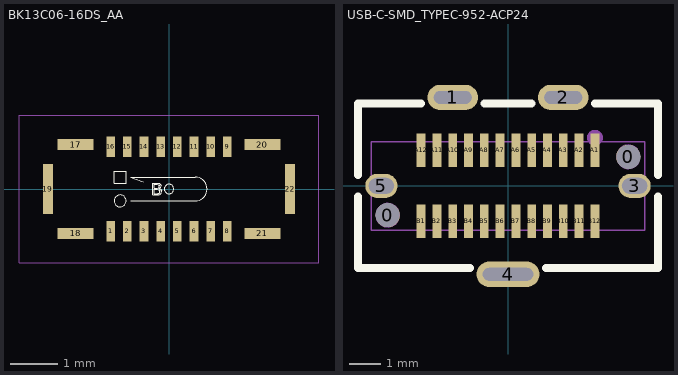
[diagram p0: the footprints below, top view; thin cyan lines are the x and y axes]
# Altium footprint library MISC89352.PcbLib: 2 footprints
Each footprint in its own frame and in the unit in brackets; x right, y up, seen from the top. Pads: shape width x height; smd on the part's side, far side on the other; paste and mask are expansions set on the pad; w line width, h text height; cw(c..) or ccw(c..) is an arc to the next point about the centre after c.

## BK13C06-16DS_AA [mm]
pads (22):
  rect 0.18x0.425 smd paste+0.102 mask+0.072: 1(-1.225,-0.887) 2(-0.875,-0.887) 3(-0.525,-0.887) 4(-0.175,-0.887) 5(0.175,-0.887) 6(0.525,-0.887) 7(0.875,-0.887) 8(1.225,-0.887) 9(1.225,0.887) 10(0.875,0.887) 11(0.525,0.887) 12(0.175,0.887) 13(-0.175,0.887) 14(-0.525,0.887) 15(-0.875,0.887) 16(-1.225,0.887)
  rect 0.75x0.235 smd paste+0.102 mask+0.05: 17(-1.96,0.932) 18(-1.96,-0.932) 20(1.96,0.932) 21(1.96,-0.932)
  rect 0.215x1.04 smd paste+0.102 mask+0.05: 19(-2.54,0) 22(2.54,0)
Top Overlay:
  circle w0.013: c-1.025,-0.25 r0.125
  circle w0.013: c0,0 r0.1
  lines w0.013: -0.8,-0.25 0.55,-0.25 ccw(c0.55,0) 0.55,0.25 -0.8,0.25 -0.537,0.155 ; -1.15,0.125 -0.9,0.125 -0.9,0.375 -1.15,0.375 -1.15,0.125 ; -0.344,-0.125 -0.237,-0.125 -0.217,-0.123 -0.209,-0.121 -0.201,-0.119 -0.187,-0.113 -0.181,-0.108 -0.176,-0.104 -0.167,-0.093 -0.159,-0.078 -0.156,-0.061 -0.156,-0.042 -0.162,-0.023 -0.168,-0.015 -0.174,-0.007 -0.191,0.005 -0.203,0.008 -0.194,0.012 -0.181,0.024 -0.176,0.031 -0.172,0.038 -0.168,0.053 -0.168,0.07 -0.173,0.086 -0.178,0.094 -0.182,0.102 -0.196,0.114 -0.205,0.117 -0.213,0.121 -0.236,0.125 -0.344,0.125 -0.344,-0.125 ; -0.311,-0.095 -0.311,-0.01 -0.242,-0.01 -0.223,-0.012 -0.217,-0.014 -0.211,-0.016 -0.201,-0.023 -0.197,-0.028 -0.193,-0.033 -0.19,-0.046 -0.19,-0.058 -0.192,-0.069 -0.195,-0.074 -0.197,-0.078 -0.204,-0.085 -0.207,-0.087 -0.211,-0.09 -0.221,-0.093 -0.227,-0.094 -0.23,-0.095 -0.241,-0.095 -0.311,-0.095 ; -0.311,0.02 -0.311,0.095 -0.248,0.095 -0.229,0.094 -0.223,0.092 -0.218,0.09 -0.209,0.084 -0.206,0.079 -0.203,0.074 -0.2,0.063 -0.2,0.051 -0.203,0.04 -0.21,0.031 -0.219,0.025 -0.226,0.023 -0.23,0.021 -0.246,0.02 -0.311,0.02
Mechanical 1:
  lines w0.013: -3.147,-1.55 3.147,-1.55 3.147,1.55 -3.147,1.55 -3.147,-1.55

## USB-C-SMD_TYPEC-952-ACP24 [mm]
pads (31):
  round 0.76 hole 0.76 unplated: 0(-3.81,-0.93) 0(3.81,0.92)
  oval 1.6x0.8 hole 0.4 slot 1.2 at 0 deg paste+0 mask+0.05: 1(-1.75,2.8) 2(1.75,2.8)
  oval 1.016x0.762 hole 0.5 slot 0.8 at 0 deg paste+0 mask+0.05: 3(4.01,0) 5(-4.01,0)
  oval 2x0.8 hole 0.4 slot 1.6 at 0 deg paste+0 mask+0.05: 4(0,-2.8)
  rect 0.28x1.06 smd paste-100 mask+0.05: A1(2.75,1.12) A2(2.25,1.12) A3(1.75,1.12) A4(1.25,1.12) A5(0.75,1.12) A6(0.25,1.12) A7(-0.25,1.12) A8(-0.75,1.12) A9(-1.25,1.12) A10(-1.75,1.12) A11(-2.25,1.12) A12(-2.75,1.12) B1(-2.75,-1.12) B2(-2.25,-1.12) B3(-1.75,-1.12) B4(-1.25,-1.12) B5(-0.75,-1.12) B6(-0.25,-1.12) B7(0.25,-1.12) B8(0.75,-1.12) B9(1.25,-1.12) B10(1.75,-1.12) B11(2.25,-1.12) B12(2.75,-1.12)
Top Overlay:
  lines w0.254: -4.75,-0.338 -4.75,-2.6 -1.198,-2.6 ; -4.75,0.338 -4.75,2.6 -2.748,2.6 ; -0.752,2.6 0.752,2.6 ; 1.198,-2.6 4.75,-2.6 4.75,-0.338 ; 2.748,2.6 4.75,2.6 4.75,0.338
Mechanical 1:
  circle w0.025: c3.81,0.92 r0.375
  circle w0.025: c-3.81,-0.93 r0.375
Mechanical 6:
  circle w0.25: c3.81,0.92 r0.125
  circle w0.25: c-3.81,-0.93 r0.125
  circle w0.25: c2.755,1.525 r0.125
Mechanical 15:
  lines w0.051: -4.33,-1.4 -4.33,1.4 4.33,1.4 4.33,-1.4 -4.33,-1.4